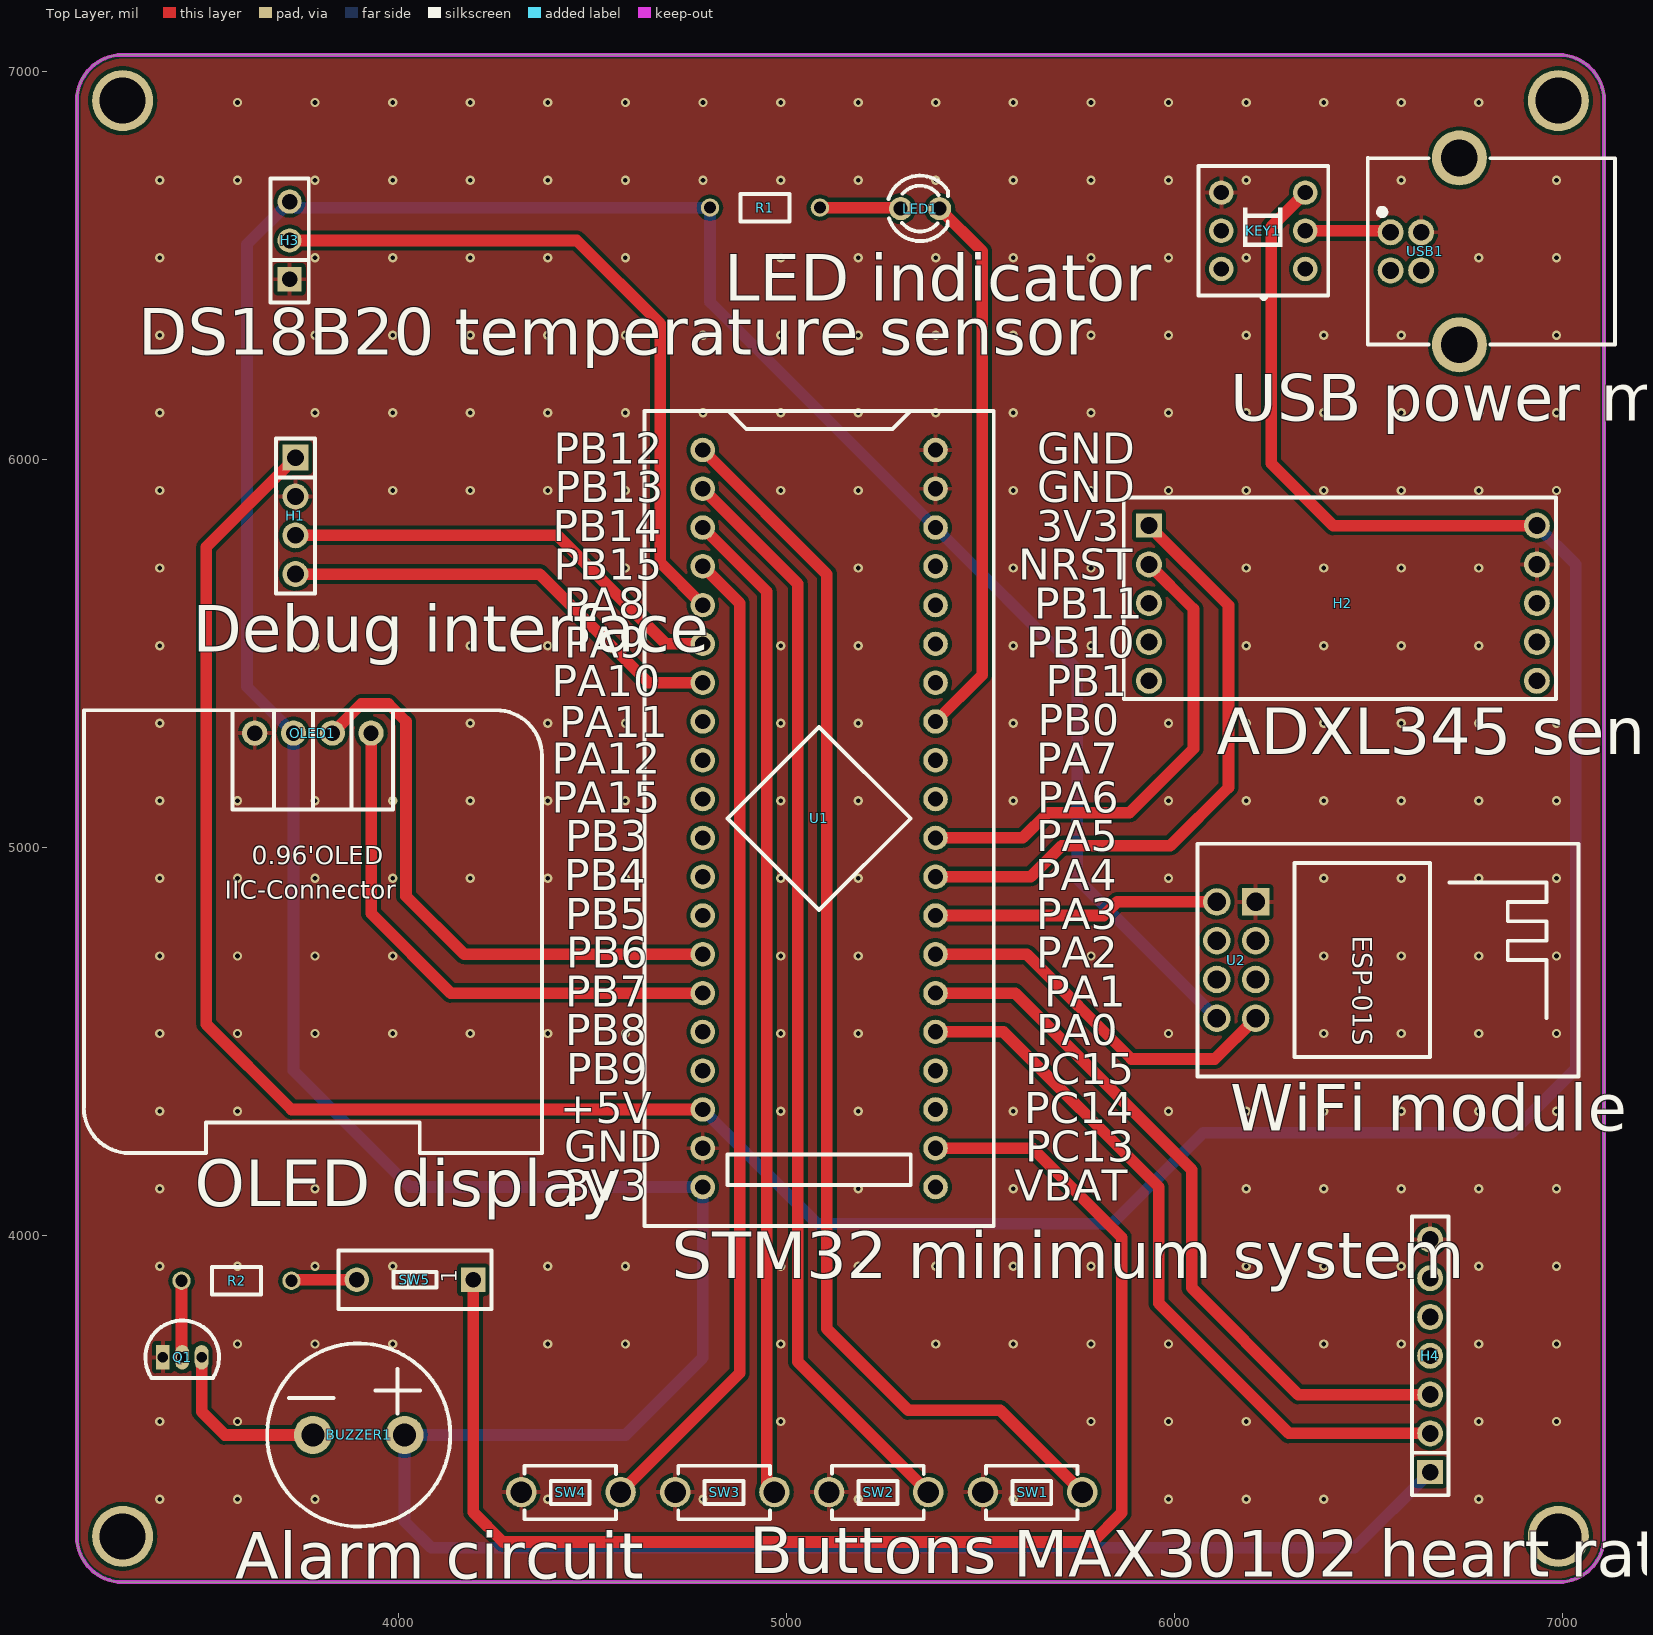
[diagram p0: Top Layer view]
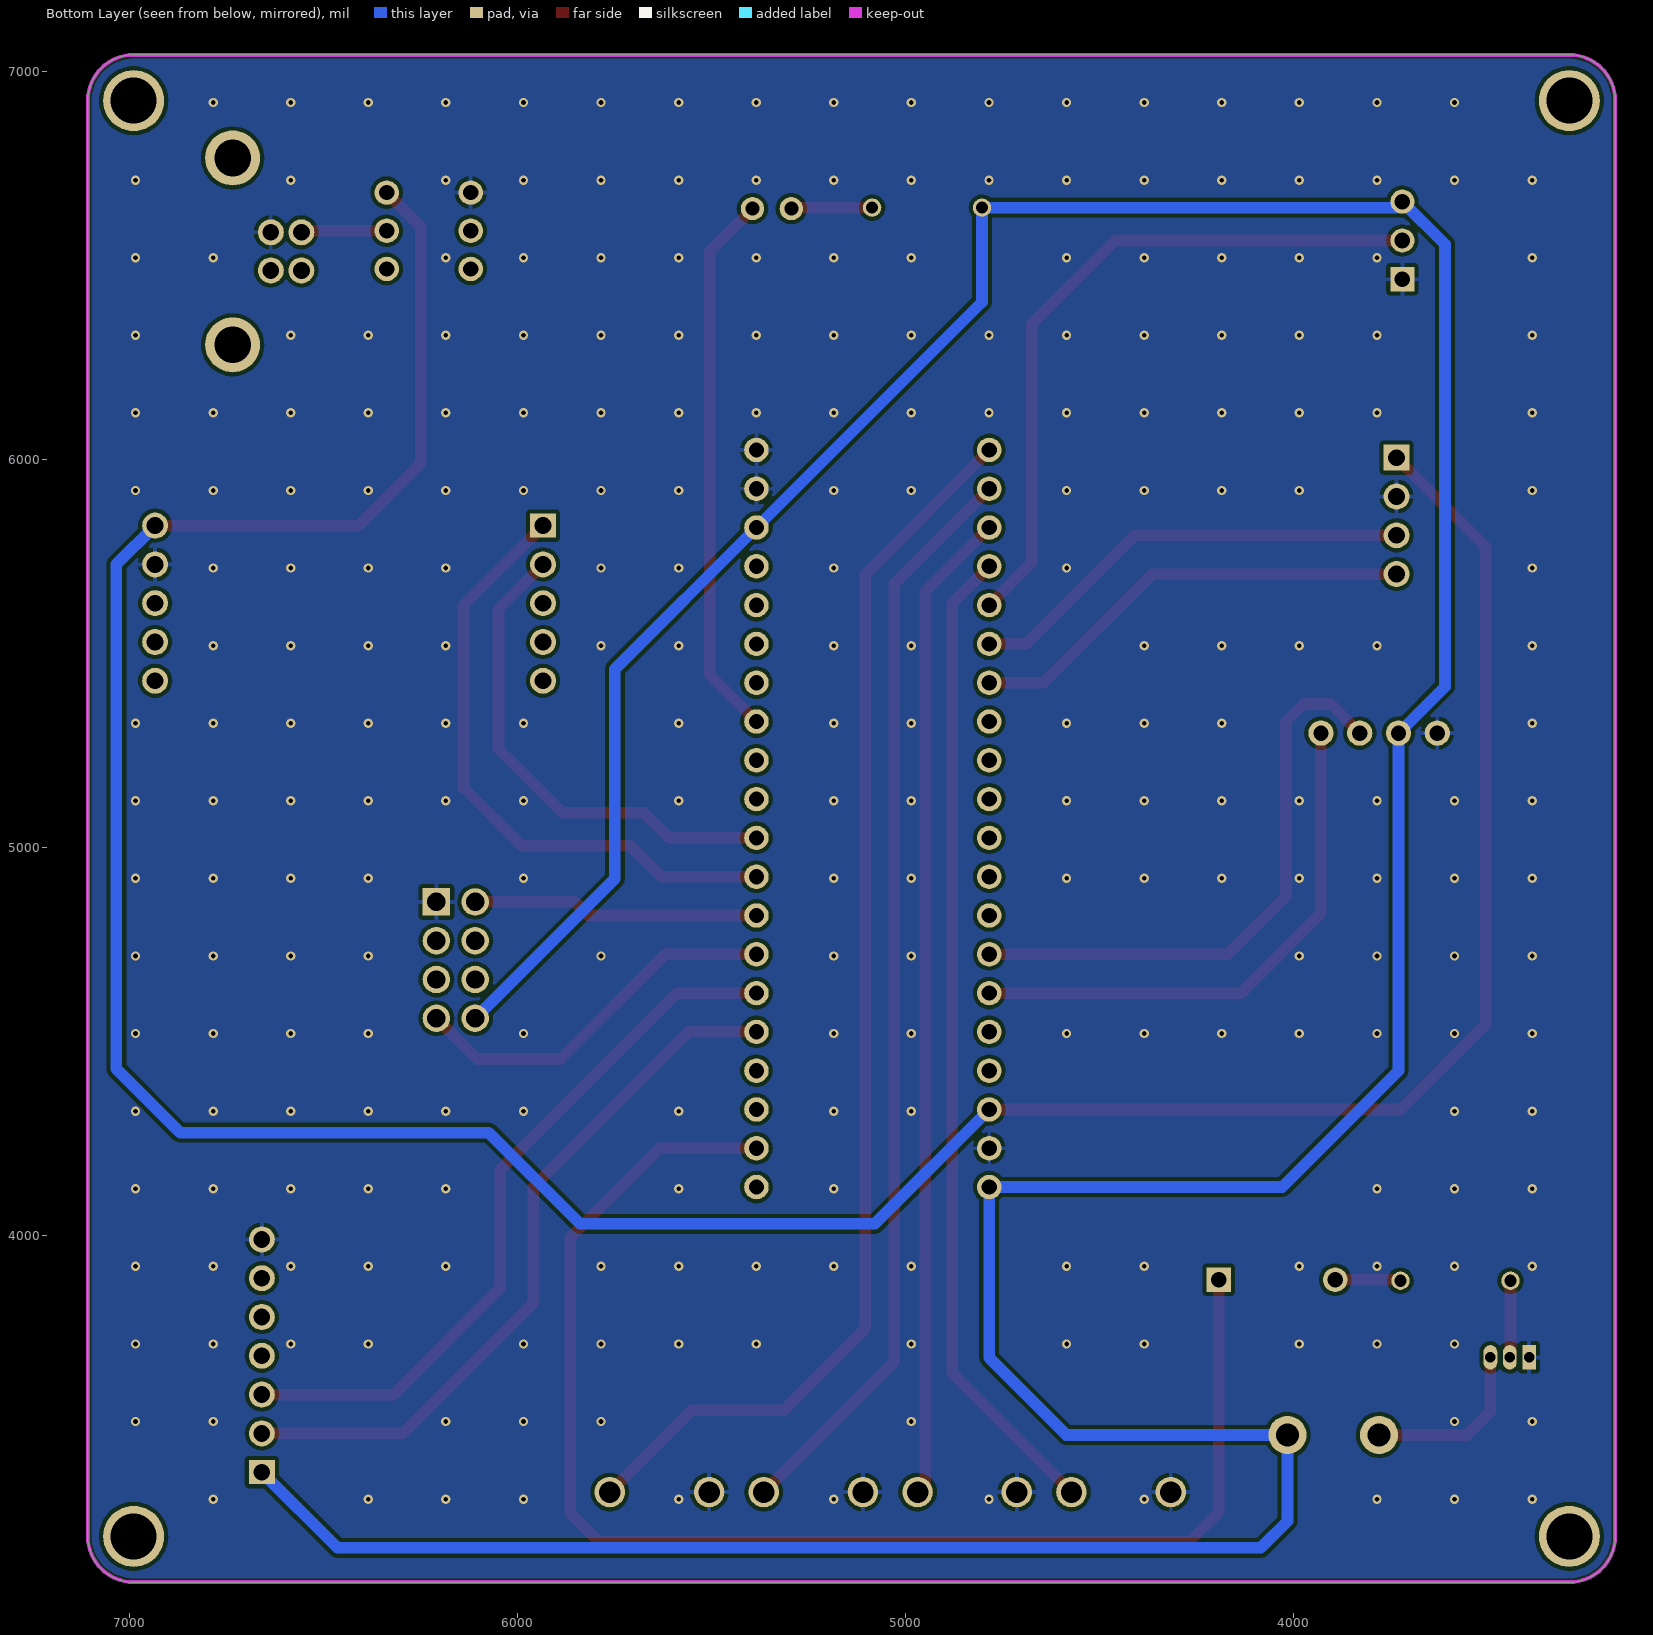
[diagram p1: Bottom Layer view, seen from below]
# Altium PCB MISC51590.pcbdoc
Units mil, origin at the board's own origin, x right, y up, seen from the top; angles counter-clockwise.
Board outline 3937.01 x 3937.01 mil, 2 copper layers (Top Layer, Bottom Layer), stack 62.206 mil thick; 19 components, 42 nets, 113 pads, 259 vias.

## Layer stack, top to bottom
Top Solder Mask Layer: solder mask 0.394, Dk 3.3
Top Layer: signal copper 1.379
Dielectric1: surface 59.449, FR4, Dk 4.5
Bottom Layer: signal copper 1.378
Bottom Solder Mask Layer: solder mask 0.394, Dk 3.3

## Board outline
6990.39,3106.5 ccw(c6990.39,3224.61) 7108.5,3224.61 7108.5,6925.39 ccw(c6990.39,6925.39) 6990.39,7043.5 3289.61,7043.5 ccw(c3289.61,6925.39) 3171.5,6925.39 3171.5,3224.61 ccw(c3289.61,3224.61) 3289.61,3106.5

## Design rules (kind name [scope] priority, off if disabled: settings)
BoardOutlineClearance copperThickness2oz_1 [All] p2 off: genericclearance=7.99 ignorepadtopadclearanceinfootprint=FALSE except(0: Arc-SplitContinuation Track-SplitContinuation SMDPad-SplitContinuation THPad-SplitContinuation Via-SplitContinuation Fill-SplitContinuation Region-SplitContinuation Poly-SplitContinuation Text-SplitContinuation Hole-SplitContinuation; 5.98: Arc-CutoutEdge Track-CutoutEdge SMDPad-CutoutEdge THPad-CutoutEdge Via-CutoutEdge Text-CutoutEdge; 6.89: Hole-OutlineEdge Hole-CutoutEdge; 10: Poly-OutlineEdge Poly-CutoutEdge; 11.81: Arc-OutlineEdge Track-OutlineEdge SMDPad-OutlineEdge THPad-OutlineEdge Via-OutlineEdge Fill-OutlineEdge Region-OutlineEdge Text-OutlineEdge Fill-CutoutEdge Region-CutoutEdge)
BoardOutlineClearance Plane_innerPlane_1 [All] p4 off: genericclearance=4.02 ignorepadtopadclearanceinfootprint=FALSE except(0: Arc-SplitContinuation Track-SplitContinuation SMDPad-SplitContinuation THPad-SplitContinuation Via-SplitContinuation Fill-SplitContinuation Region-SplitContinuation Poly-SplitContinuation Text-SplitContinuation Hole-SplitContinuation; 5.98: Arc-CutoutEdge Track-CutoutEdge SMDPad-CutoutEdge THPad-CutoutEdge Via-CutoutEdge Text-CutoutEdge; 6.89: Hole-OutlineEdge Hole-CutoutEdge; 10: Poly-OutlineEdge Poly-CutoutEdge; 11.81: Arc-OutlineEdge Track-OutlineEdge SMDPad-OutlineEdge THPad-OutlineEdge Via-OutlineEdge Fill-OutlineEdge Region-OutlineEdge Text-OutlineEdge Fill-CutoutEdge Region-CutoutEdge)
BoardOutlineClearance Copper_copperRegion_1 [All] p6 off: genericclearance=4.02 ignorepadtopadclearanceinfootprint=FALSE except(0: Arc-SplitContinuation Track-SplitContinuation SMDPad-SplitContinuation THPad-SplitContinuation Via-SplitContinuation Fill-SplitContinuation Region-SplitContinuation Poly-SplitContinuation Text-SplitContinuation Hole-SplitContinuation; 5.98: Arc-CutoutEdge Track-CutoutEdge SMDPad-CutoutEdge THPad-CutoutEdge Via-CutoutEdge Text-CutoutEdge; 6.89: Hole-OutlineEdge Hole-CutoutEdge; 10: Poly-OutlineEdge Poly-CutoutEdge; 11.81: Arc-OutlineEdge Track-OutlineEdge SMDPad-OutlineEdge THPad-OutlineEdge Via-OutlineEdge Fill-OutlineEdge Region-OutlineEdge Text-OutlineEdge Fill-CutoutEdge Region-CutoutEdge)
BoardOutlineClearance copperThickness1oz_1 [All] p8: genericclearance=4.02 ignorepadtopadclearanceinfootprint=FALSE except(0: Arc-SplitContinuation Track-SplitContinuation SMDPad-SplitContinuation THPad-SplitContinuation Via-SplitContinuation Fill-SplitContinuation Region-SplitContinuation Poly-SplitContinuation Text-SplitContinuation Hole-SplitContinuation; 5.98: Arc-CutoutEdge Track-CutoutEdge SMDPad-CutoutEdge THPad-CutoutEdge Via-CutoutEdge Text-CutoutEdge; 6.89: Hole-OutlineEdge Hole-CutoutEdge; 10: Poly-OutlineEdge Poly-CutoutEdge; 11.81: Arc-OutlineEdge Track-OutlineEdge SMDPad-OutlineEdge THPad-OutlineEdge Via-OutlineEdge Fill-OutlineEdge Region-OutlineEdge Text-OutlineEdge Fill-CutoutEdge Region-CutoutEdge)
Clearance copperThickness2oz [All] p1 off: gap=7.99 ignorepadtopadclearanceinfootprint=FALSE except(5.98: SMDPad-Track SMDPad-SMDPad THPad-Track SMDPad-THPad THPad-THPad Track-Via SMDPad-Via THPad-Via Via-Via Fill-SMDPad Region-SMDPad Fill-THPad Region-THPad Fill-Via Region-Via Fill-Fill Fill-Region Region-Region Arc-Track Arc-SMDPad Arc-THPad Arc-Via Fill-Arc Region-Arc Arc-Arc Text-Track SMDPad-Text Text-THPad Text-Via Fill-Text Region-Text Arc-Text Text-Text; 6.89: Hole-Track Hole-SMDPad Hole-THPad Hole-Via Fill-Hole Region-Hole Hole-Arc Hole-Text; 10: Poly-Track Poly-SMDPad Poly-THPad Poly-Via Poly-Fill Poly-Region Poly-Poly Poly-Arc Poly-Text Poly-Hole; 11.81: Fill-Track Region-Track)
Clearance Plane_innerPlane [All] p3 off: gap=4.02 ignorepadtopadclearanceinfootprint=FALSE except(5.98: SMDPad-Track SMDPad-SMDPad THPad-Track SMDPad-THPad THPad-THPad Track-Via SMDPad-Via THPad-Via Via-Via Fill-SMDPad Region-SMDPad Fill-THPad Region-THPad Fill-Via Region-Via Fill-Fill Fill-Region Region-Region Arc-Track Arc-SMDPad Arc-THPad Arc-Via Fill-Arc Region-Arc Arc-Arc Text-Track SMDPad-Text Text-THPad Text-Via Fill-Text Region-Text Arc-Text Text-Text; 6.89: Hole-Track Hole-SMDPad Hole-THPad Hole-Via Fill-Hole Region-Hole Hole-Arc Hole-Text; 10: Poly-Track Poly-SMDPad Poly-THPad Poly-Via Poly-Fill Poly-Region Poly-Poly Poly-Arc Poly-Text Poly-Hole; 11.81: Fill-Track Region-Track)
Clearance Copper_copperRegion [All] p5 off: gap=4.02 ignorepadtopadclearanceinfootprint=FALSE except(5.98: SMDPad-Track SMDPad-SMDPad THPad-Track SMDPad-THPad THPad-THPad Track-Via SMDPad-Via THPad-Via Via-Via Fill-SMDPad Region-SMDPad Fill-THPad Region-THPad Fill-Via Region-Via Fill-Fill Fill-Region Region-Region Arc-Track Arc-SMDPad Arc-THPad Arc-Via Fill-Arc Region-Arc Arc-Arc Text-Track SMDPad-Text Text-THPad Text-Via Fill-Text Region-Text Arc-Text Text-Text; 6.89: Hole-Track Hole-SMDPad Hole-THPad Hole-Via Fill-Hole Region-Hole Hole-Arc Hole-Text; 10: Poly-Track Poly-SMDPad Poly-THPad Poly-Via Poly-Fill Poly-Region Poly-Poly Poly-Arc Poly-Text Poly-Hole; 11.81: Fill-Track Region-Track)
Clearance copperThickness1oz [All] p7: gap=4.02 ignorepadtopadclearanceinfootprint=FALSE except(5.98: SMDPad-Track SMDPad-SMDPad THPad-Track SMDPad-THPad THPad-THPad Track-Via SMDPad-Via THPad-Via Via-Via Fill-SMDPad Region-SMDPad Fill-THPad Region-THPad Fill-Via Region-Via Fill-Fill Fill-Region Region-Region Arc-Track Arc-SMDPad Arc-THPad Arc-Via Fill-Arc Region-Arc Arc-Arc Text-Track SMDPad-Text Text-THPad Text-Via Fill-Text Region-Text Arc-Text Text-Text; 6.89: Hole-Track Hole-SMDPad Hole-THPad Hole-Via Fill-Hole Region-Hole Hole-Arc Hole-Text; 10: Poly-Track Poly-SMDPad Poly-THPad Poly-Via Poly-Fill Poly-Region Poly-Poly Poly-Arc Poly-Text Poly-Hole; 11.81: Fill-Track Region-Track)
DiffPairsRouting differentialPair [All] p1: maxlimit=6 minlimit=6 mostfreqgap=6 toplayer_minwidth=5 toplayer_prefwidth=10 toplayer_maxwidth=100 toplayer_mingap=6 toplayer_prefgap=6 toplayer_maxgap=6 bottomlayer_minwidth=5 bottomlayer_prefwidth=10 bottomlayer_maxwidth=100 bottomlayer_mingap=6 bottomlayer_prefgap=6 bottomlayer_maxgap=6 maxuncoupledlength=10
HoleToHoleClearance otherClearance [All] p1: gap=11.81 allowstackedmicrovias=TRUE
Length netLength [All] p1: minlimit=0 maxlimit=0
PasteMaskExpansion pasteMaskExpansion [All] p1: expansion=0
PlaneConnect innerPlane [All] p1: planeconnectstyle=Relief reliefexpansion=20 reliefentries=4 reliefconductorwidth=10 reliefairgap=10
PolygonConnect copperRegion [All] p1: connectstyle=Relief reliefconductorwidth=10 reliefentries=4 polygonreliefangle="90 Angle" airgapwidth=10 via.connectstyle=Relief via.reliefconductorwidth=10 via.reliefentries=4 via.polygonreliefangle="90 Angle" via.airgapwidth=10
RoutingVias viaSize [All] p1: holewidth=12.01 width=24.02 viastyle="Through Hole" minholewidth=11.81 minwidth=19.68 maxholewidth=248.03 maxwidth=393.7
SolderMaskExpansion solderMaskExpansion [IsVia] p1: expansion=-1000 istentingtop=TRUE
SolderMaskExpansion solderMaskExpansion [All] p2: expansion=2.01 istentingtop=FALSE
Width copperThickness2oz_2 [All] p1 off: maxlimit=100 minlimit=8 preferedwidth=10
Width copperThickness1oz_2 [All] p2: maxlimit=100 minlimit=5 preferedwidth=30

## Components (designator, comment, footprint, x,y, rotation, side; value= is the part's Value field where it differs from the comment)
BUZZER1 "buzzer" BUZ-TH_BD12.0-P6.00-D0.9-RD 3898.15,3486.01 r0 top
H1 "" HDR-TH_4P-P2.54-V-M 3735,5855 r270 top
H2 "" HDR-TH_10P-P2.54-V-F-R2-C5-S2.54 5935,5630 r270 top
H3 "" HDR-TH_3P-P2.54-V-F 3720,6565 r90 top
H4 "" HDR-TH_7P-P2.54-V-F 6660,3690 r90 top
KEY1 "Non-self-locking switch 8.5×8.5 silent" SW-TH_6P-L8.5-W8.5-P2.54 6230,6590 r90 top
LED1 "" LED_TH-3mm 5345.2,6647.2 r0 top
OLED1 "" 0.96OLED_4P 3780,5295 r0 top
Q1 "" S8050_TO_92 3443.15,3686.01 r0 top
R1 "220" Res_1/8W 4945.2,6647.2 r0 top
R2 "10kΩ" Res_1/8W 3583.15,3886.01 r180 top
SW1 "" Key_TH_3.5x6x4.3 5628.58,3338.7 r0 top
SW2 "" Key_TH_3.5x6x4.3 5231.92,3338.7 r0 top
SW3 "" Key_TH_3.5x6x4.3 4835.25,3338.7 r0 top
SW4 "" Key_TH_3.5x6x4.3 4438.58,3338.7 r0 top
SW5 "NDS-01V" SW-TH_2P-L3.9-W9.9-P2.54-LS7.6 4043.15,3886.01 r180 top
U1 "STM32F103C8T6-Card" CONN-TH_L53.3-W22.9_STM32F103C8T6-CARD 5085,5075 r270 top
U2 "ESP-01S" WIFIM-TH_ESP-01S 6160,4710 r270 top
USB1 "" "USB_ Type-B" 6815.29,6531.4 r90 top

## Footprints (in the part's own frame and the unit in brackets; to place one, negate y for a bottom-side part, rotate by r counter-clockwise, add the part's x,y. Pads: shape width x height; smd on the part's side, far side on the other; paste and mask are expansions set on the pad)
0.96OLED_4P [mm]
  round 1.65 hole 1 copper offset 0,0: 1(-3.81,-0.001) 2(-1.27,0.002) 3(1.27,0.002) 4(3.81,0.002)
  silkscreen extent -15,-27.5 15,1.5
BUZ-TH_BD12.0-P6.00-D0.9-RD [mm]
  round 2.5 hole 1.5 paste+0 mask+0.05: 1(-3,0) 2(3,0)
  silkscreen extent -5.99,-5.99 5.99,5.99
CONN-TH_L53.3-W22.9_STM32F103C8T6-CARD [mm]
  round 1.6 hole 1: 1(-24.13,-7.62) 2(-21.59,-7.62) 3(-19.05,-7.62) 4(-16.51,-7.62) 5(-13.97,-7.62) 6(-11.43,-7.62) 7(-8.89,-7.62) 8(-6.35,-7.62) 9(-3.81,-7.62) 10(-1.27,-7.62) 11(1.27,-7.62) 12(3.81,-7.62) 13(6.35,-7.62) 14(8.89,-7.62) 15(11.43,-7.62) 16(13.97,-7.62) 17(16.51,-7.62) 18(19.05,-7.62) 19(21.59,-7.62) 20(24.13,-7.62) 21(24.13,7.62) 22(21.59,7.62) 23(19.05,7.62) 24(16.51,7.62) 25(13.97,7.62) 26(11.43,7.62) 27(8.89,7.62) 28(6.35,7.62) 29(3.81,7.62) 30(1.27,7.62) 31(-1.27,7.62) 32(-3.81,7.62) 33(-6.35,7.62) 34(-8.89,7.62) 35(-11.43,7.62) 36(-13.97,7.62) 37(-16.51,7.62) 38(-19.05,7.62) 39(-21.59,7.62) 40(-24.13,7.62)
  silkscreen extent -26.67,-11.43 26.67,11.43
HDR-TH_3P-P2.54-V-F [mil]
  rect 62x62 hole 40.16: 1(-100,0)
  round 62 hole 40.16: 2(0,0) 3(100,0)
  silkscreen extent -160,-49 160,49
HDR-TH_4P-P2.54-V-M [mm]
  rect 1.7x1.7 hole 1.1: 1(-3.81,0)
  round 1.7 hole 1.1: 2(-1.27,0) 3(1.27,0) 4(3.81,0)
  silkscreen extent -5.08,-1.27 5.08,1.27
HDR-TH_7P-P2.54-V-F [mm]
  rect 1.575x1.7 hole 1.1: 1(-7.62,0)
  round 1.7 hole 1.1: 2(-5.08,0) 3(-2.54,0) 4(0,0) 5(2.54,0) 6(5.08,0) 7(7.62,0)
  silkscreen extent -9.13,-1.2 9.13,1.2
HDR-TH_10P-P2.54-V-F-R2-C5-S2.54 [mm]
  rect 1.575x1.7 hole 1.1: 1(-5.08,0)
  round 1.7 hole 1.1: 2(-5.08,25.4) 3(-2.54,0) 4(-2.54,25.4) 5(0,0) 6(0,25.4) 7(2.54,0) 8(2.54,25.4) 9(5.08,0) 10(5.08,25.4)
  silkscreen extent -6.93,-1.65 6.27,26.65
Key_TH_3.5x6x4.3 [mil]
  round 78.7 hole 55.1 paste+0 mask+2: A(-121.44,0) B(134.46,0)
  silkscreen extent -114,-70 123,68
LED_TH-3mm [mil]
  round 60 hole 36 paste+0 mask+2: 1(-50,0) 2(50,0)
  silkscreen extent -81,-84 72,85
Res_1/8W [mil]
  round 47.2 hole 31.5 paste+0 mask+2: 1(-141.7,2.48) 2(141.7,2.48)
  silkscreen extent -63,-33 63,38
S8050_TO_92 [mil]
  rect 35.4x63 hole 27.6 paste+0 mask+2: 1(-50,0)
  oval 35.4x63 hole 27.6 paste+0 mask+2: 2(0,0) 3(50,0)
  silkscreen extent -95,-53 95,95
SW-TH_2P-L3.9-W9.9-P2.54-LS7.6 [mm]
  rect 1.6x1.6 hole 1 paste+0 mask+0.05: 1(-3.81,0)
  round 1.6 hole 1 paste+0 mask+0.05: 2(3.81,0)
  silkscreen extent -5,-1.91 5,1.91
SW-TH_6P-L8.5-W8.5-P2.54 [mm]
  round 1.6 hole 1: 1(-2.5,-2.75) 2(0,-2.75) 3(2.5,-2.75) 4(-2.5,2.75) 5(0,2.75) 6(2.5,2.75)
  silkscreen extent -4.47,-4.25 4.25,4.25
"USB_ Type-B" [mm]
  round 1.7 hole 1.1 copper offset 0,0 paste+0 mask+0.051: 1(1.39,6.532) 2(-1.11,6.532) 3(-1.11,4.532) 4(1.39,4.532)
  round 3.6 hole 2.4 paste+0 mask+0.051: 5(-5.977,2.032) 5(6.256,2.032)
  silkscreen extent -5.96,-8.17 6.25,8.03
WIFIM-TH_ESP-01S [mm]
  rect 1.8x1.8 hole 1.2: 1(-3.81,1.27)
  round 1.8 hole 1.2: 2(-1.27,1.27) 3(1.27,1.27) 4(3.81,1.27) 5(3.81,-1.27) 6(1.27,-1.27) 7(-1.27,-1.27) 8(-3.81,-1.27)
  silkscreen extent -7.62,-2.54 7.62,22.4

## Free pads (board coordinates)
  round 157.48 hole 118.11: 1(3289.61,6925.39) 1(3289.61,3224.61) 1(6990.39,6925.39) 1(6990.39,3224.61)

## Via types
v1: diameter 24.02, hole 12, Top Layer to Bottom Layer, 259 vias

## Nets (pads, with @x,y where several pads share a name; then routed paths per layer and width w, separated by ;. In a path a pad name is that pad's centre, name@x,y a point inside that pad or via, vN(x,y) a via of type N, cw(c..) or ccw(c..) an arc to the next point about the centre after c; other vN are vias at no path point)
$1N18282: KEY1.2 USB1.1 | length 221.5
  Top Layer w30: KEY1.2 6554.25,6589.99 USB1.1
$1N18294: LED1.1 R1.2 | length 209.3
  Top Layer w30: R1.2 5292.72,6649.68 LED1.1
$1N18316: BUZZER1.1 Q1.3 | length 451.7
  Top Layer w30: Q1.3 3493.15,3546.01 3553.15,3486.01 BUZZER1.1
$1N18318: R2.1 SW5.2 | length 169.3
  Top Layer w30: R2.1 3727.32,3886.01 SW5.2
$1N18319: Q1.2 R2.2 | length 198.2
  Top Layer w30: R2.2 3441.45,3687.71 Q1.2
+5V: H1.1 H2.2 KEY1.3 U1.18 | length 8392
  Top Layer w30: H1.1 3505,5775 3505,4545 3725,4325 U1.18 ; KEY1.3 6250,6600.15 6250,5990 6410,5830 H2.2
  Bottom Layer w30: U1.18 5080,4030 5840,4030 6075,4265 6870,4265 7035,4430 7035,5730 H2.2
GND: H1.2 H2.4 H3.1 H4.7 KEY1.6 OLED1.1 Q1.1 SW1.A SW2.A SW3.A SW4.A U1.19 U1.39 U1.40 U2.1 USB1.4
  other v1: 3385.6,3320.6 3585.6,3320.6 3785.6,3320.6 4385.6,3320.6 4785.6,3320.6 5185.6,3320.6 5585.6,3320.6 5985.6,3320.6 6185.6,3320.6 6385.6,3320.6 6785.6,3320.6 3385.6,3520.6 3585.6,3520.6 4985.6,3520.6 5785.6,3520.6 5985.6,3520.6 6185.6,3520.6 6785.6,3520.6 6985.6,3520.6 3585.6,3720.6 3785.6,3720.6 3985.6,3720.6 4385.6,3720.6 4585.6,3720.6 4985.6,3720.6 5385.6,3720.6 5585.6,3720.6 5785.6,3720.6 5985.6,3720.6 6385.6,3720.6 6585.6,3720.6 6785.6,3720.6 6985.6,3720.6 3385.6,3920.6 3585.6,3920.6 3785.6,3920.6 3985.6,3920.6 4385.6,3920.6 4585.6,3920.6 4985.6,3920.6 5185.6,3920.6 5385.6,3920.6 5585.6,3920.6 5785.6,3920.6 6185.6,3920.6 6385.6,3920.6 6585.6,3920.6 6785.6,3920.6 6985.6,3920.6 3385.6,4120.6 3585.6,4120.6 3785.6,4120.6 5185.6,4120.6 5585.6,4120.6 6185.6,4120.6 6385.6,4120.6 6585.6,4120.6 6785.6,4120.6 6985.6,4120.6 3385.6,4320.6 3585.6,4320.6 4985.6,4320.6 5185.6,4320.6 5585.6,4320.6 5985.6,4320.6 6185.6,4320.6 6385.6,4320.6 6585.6,4320.6 6785.6,4320.6 6985.6,4320.6 3385.6,4520.6 3585.6,4520.6 3785.6,4520.6 3985.6,4520.6 4185.6,4520.6 4385.6,4520.6 4585.6,4520.6 4985.6,4520.6 5185.6,4520.6 5985.6,4520.6 6385.6,4520.6 6585.6,4520.6 6785.6,4520.6 6985.6,4520.6 3385.6,4720.6 3585.6,4720.6 3785.6,4720.6 3985.6,4720.6 4985.6,4720.6 5185.6,4720.6 5785.6,4720.6 6385.6,4720.6 6585.6,4720.6 6785.6,4720.6 6985.6,4720.6 3385.6,4920.6 3585.6,4920.6 3785.6,4920.6 3985.6,4920.6 4185.6,4920.6 4385.6,4920.6 4585.6,4920.6 4985.6,4920.6 5185.6,4920.6 5985.6,4920.6 6385.6,4920.6 6585.6,4920.6 6785.6,4920.6 6985.6,4920.6 3385.6,5120.6 3585.6,5120.6 3785.6,5120.6 3985.6,5120.6 4185.6,5120.6 4385.6,5120.6 4585.6,5120.6 4985.6,5120.6 5185.6,5120.6 5585.6,5120.6 5985.6,5120.6 6185.6,5120.6 6385.6,5120.6 6585.6,5120.6 6785.6,5120.6 6985.6,5120.6 3385.6,5320.6 4185.6,5320.6 4385.6,5320.6 4585.6,5320.6 4985.6,5320.6 5185.6,5320.6 5585.6,5320.6 5985.6,5320.6 6185.6,5320.6 6385.6,5320.6 6585.6,5320.6 6785.6,5320.6 6985.6,5320.6 3385.6,5520.6 3785.6,5520.6 3985.6,5520.6 4185.6,5520.6 4385.6,5520.6 4985.6,5520.6 5185.6,5520.6 5585.6,5520.6 5785.6,5520.6 6185.6,5520.6 6385.6,5520.6 6585.6,5520.6 6785.6,5520.6 3385.6,5720.6 4585.6,5720.6 5185.6,5720.6 5585.6,5720.6 5785.6,5720.6 6185.6,5720.6 6385.6,5720.6 6585.6,5720.6 6785.6,5720.6 3385.6,5920.6 3985.6,5920.6 4185.6,5920.6 4385.6,5920.6 4585.6,5920.6 4985.6,5920.6 5185.6,5920.6 5585.6,5920.6 5785.6,5920.6 5985.6,5920.6 6185.6,5920.6 6385.6,5920.6 6585.6,5920.6 6785.6,5920.6 6985.6,5920.6 3385.6,6120.6 3785.6,6120.6 3985.6,6120.6 4185.6,6120.6 4385.6,6120.6 4585.6,6120.6 4785.6,6120.6 4985.6,6120.6 5185.6,6120.6 5385.6,6120.6 5585.6,6120.6 5785.6,6120.6 5985.6,6120.6 6185.6,6120.6 6385.6,6120.6 6585.6,6120.6 6785.6,6120.6 6985.6,6120.6 3385.6,6320.6 3785.6,6320.6 3985.6,6320.6 4185.6,6320.6 4385.6,6320.6 4585.6,6320.6 4785.6,6320.6 4985.6,6320.6 5185.6,6320.6 5385.6,6320.6 5585.6,6320.6 5785.6,6320.6 5985.6,6320.6 6185.6,6320.6 6385.6,6320.6 6585.6,6320.6 6985.6,6320.6 3385.6,6520.6 3785.6,6520.6 3985.6,6520.6 4185.6,6520.6 4385.6,6520.6 4585.6,6520.6 4985.6,6520.6 5185.6,6520.6 5385.6,6520.6 5585.6,6520.6 5785.6,6520.6 5985.6,6520.6 6185.6,6520.6 6785.6,6520.6 6985.6,6520.6 3385.6,6720.6 3585.6,6720.6 3785.6,6720.6 3985.6,6720.6 4185.6,6720.6 4385.6,6720.6 4585.6,6720.6 4785.6,6720.6 4985.6,6720.6 5185.6,6720.6 5385.6,6720.6 5585.6,6720.6 5785.6,6720.6 5985.6,6720.6 6185.6,6720.6 6585.6,6720.6 6985.6,6720.6 3585.6,6920.6 3785.6,6920.6 3985.6,6920.6 4185.6,6920.6 4385.6,6920.6 4585.6,6920.6 4785.6,6920.6 4985.6,6920.6 5185.6,6920.6 5385.6,6920.6 5585.6,6920.6 5785.6,6920.6 5985.6,6920.6 6185.6,6920.6 6385.6,6920.6 6585.6,6920.6 6785.6,6920.6
NRST: U1.37
PA0: H4.2 U1.25 | length 1879.4
  Top Layer w30: U1.25 5560,4525 5960,4125 5960,3825 6295,3490 H4.2
PA1: H4.3 U1.26 | length 1882.4
  Top Layer w30: U1.26 5590,4625 6045,4170 6045,3865 6320,3590 H4.3
PA2: U1.27 U2.4 | length 980.3
  Top Layer w30: U1.27 5620,4725 5890,4455 6105,4455 U2.4
PA3: U1.28 U2.8 | length 739.5
  Top Layer w30: U1.28 5818.51,4825 5853.51,4860 U2.8
PA4: H2.1 U1.29 | length 1610.2
  Top Layer w30: U1.29 5630,4925 5710,5005 5990,5005 6140,5155 6140,5625 H2.1
PA5: H2.3 U1.30 | length 1282.9
  Top Layer w30: U1.30 5610,5025 5675,5090 5885,5090 6050,5255 6050,5615 H2.3
PA6: U1.31
PA7: U1.32
PA8: H3.2 U1.5 | length 1814.6
  Top Layer w30: H3.2 4460,6565 4675,6350 4675,5735 U1.5
PA9: H1.3 U1.6 | length 1166
  Top Layer w30: H1.3 4410,5805 4690,5525 U1.6
PA10: H1.4 U1.7 | length 1166
  Top Layer w30: H1.4 4365,5705 4645,5425 U1.7
PA11: U1.8
PA12: U1.9
PA15: U1.10
PB0: LED1.2 U1.33 | length 1417.4
  Top Layer w30: U1.33 5505,5445 5505,6537.4 LED1.2
PB1: U1.34
PB3: U1.11
PB4: U1.12
PB5: U1.13
PB6: OLED1.3 U1.14 | length 1516.8
  Top Layer w30: OLED1.3@3830,5295.05 3904.95,5370 3975,5370 4020,5325 4020,4875 4170,4725 U1.14
PB7: OLED1.4 U1.15 | length 1405
  Top Layer w30: OLED1.4@3930,5295.05 3930,4830 4135,4625 U1.15
PB8: U1.16
PB9: U1.17
PB10: U1.35
PB11: U1.36
PB12: SW1.B U1.1 | length 3230.1
  Top Layer w30: U1.1 5105,5705 5105,3760 5315,3550 5551.74,3550 SW1.B
PB13: SW2.B U1.2 | length 2827.1
  Top Layer w30: U1.2 5030,5680 5030,3675.07 SW2.B
PB14: SW3.B U1.3 | length 2562.8
  Top Layer w30: U1.3 4950,5660 4950,3358.41 SW3.B
PB15: SW4.B U1.4 | length 2552.8
  Top Layer w30: SW4.B 4880,3645.66 4880,5630 U1.4
PC13: SW5.1 U1.22 | length 3619.2
  Top Layer w30: SW5.1 4193.15,3286.85 4270,3210 5790,3210 5865,3285 5865,3995 5635,4225 U1.22
PC14: U1.23
PC15: U1.24
VBAT: U1.21
VCC: BUZZER1.2 H3.3 H4.1 OLED1.2 R1.1 U1.20 U1.38 U2.5 | length 11501.7
  Bottom Layer w30: U2.5 5750,4920 5750,5460 U1.38 4803.5,6406.5 R1.1 3735.32,6649.68 H3.3 3610,6555 3610,5415.05 3730,5295.05 3730,4425 4030,4125 U1.20 4785,3685 4586.01,3486.01 BUZZER1.2 4016.26,3263.74 4085,3195 6465,3195 H4.1
pads on no net: H2.5 H2.6 H2.7 H2.8 H2.9 H2.10 H4.4 H4.5 H4.6 KEY1.1 KEY1.4 KEY1.5 U2.2 U2.3 U2.6 U2.7 USB1.2 USB1.3 USB1.5

## Polygon pours and split planes (outlines as drawn)
GND on Bottom Layer (solid, remove dead copper, pour order 2): 3100,7165 3100,3000 7275,3000 7275,7165
GND on Top Layer (solid, remove dead copper, pour order 0): 3000,7145 3000,3075 7385,3075 7385,7145

## Keep-outs
Board Outline Layer:
  the board outline again, w10

## Silkscreen, mask and mechanical layers (free items; w line width, h text height)
Top Silkscreen Layer:
  text "LED indicator" at 4840,6410 h120
  text "DS18B20 temperature sensor" at 3330,6270 h120
  text "USB power module" at 6145,6100 h120
  text "PB12" at 4400.64,5990 h80
  text "GND" at 5646.65,5990 h80
  text "PB13" at 4403.85,5890 h80
  text "GND" at 5646.65,5890 h80
  text "PB14" at 4398.34,5790 h80
  text "3V3" at 5644.45,5790 h80
  text "PB15" at 4400.64,5690 h80
  text "NRST" at 5598.65,5690 h80
  text "PA8" at 4426.24,5590 h80
  text "PB11" at 5639.05,5590 h80
  text "Debug interface" at 3470,5505 h120
  text "PA9" at 4428.44,5490 h80
  text "PB10" at 5618.85,5490 h80
  text "PA10" at 4396.14,5390 h80
  text "PB1" at 5669.15,5390 h80
  text "PB0" at 5648.95,5290 h80
  text "PA11" at 4414.55,5285 h80
  text "ADXL345 sensor" at 6110,5240 h120
  text "PA12" at 4396.14,5190 h80
  text "PA7" at 5644.45,5190 h80
  text "PA15" at 4396.14,5090 h80
  text "PA6" at 5646.65,5090 h80
  text "PB3" at 4430.74,4990 h80
  text "PA5" at 5644.45,4990 h80
  text "PB4" at 4428.44,4890 h80
  text "PA4" at 5642.15,4890 h80
  text "PB5" at 4430.74,4790 h80
  text "PA3" at 5644.45,4790 h80
  text "PB6" at 4432.94,4690 h80
  text "PA2" at 5644.45,4690 h80
  text "PB7" at 4430.74,4590 h80
  text "PA1" at 5664.65,4590 h80
  text "PB8" at 4430.74,4490 h80
  text "PA0" at 5644.45,4490 h80
  text "PB9" at 4432.94,4390 h80
  text "PC15" at 5616.55,4390 h80
  text "+5V" at 4417.24,4290 h80
  text "PC14" at 5614.25,4290 h80
  text "WiFi module" at 6145,4270 h120
  text "GND" at 4428.44,4190 h80
  text "PC13" at 5616.55,4190 h80
  text "3V3" at 4426.24,4090 h80
  text "VBAT" at 5589.65,4090 h80
  text "OLED display" at 3475,4075 h120
  text "STM32 minimum system" at 4705,3890 h120
  text "Buttons" at 4905,3130 h120
  text "MAX30102 heart rate and SpO2 sensor" at 5585,3120 h120
  text "Alarm circuit" at 3580,3115 h120